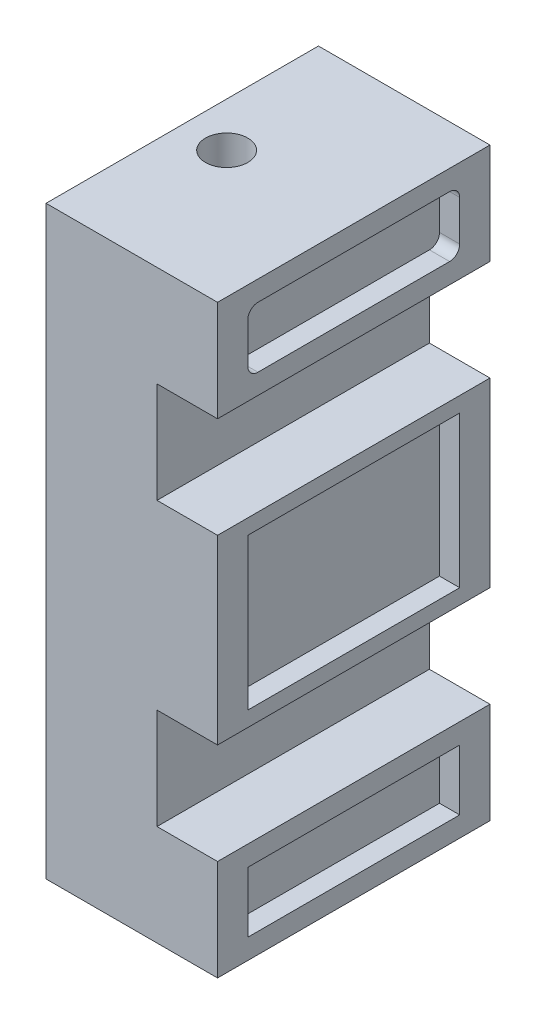
SolidWorks part; units mm, degrees
ref_plane "前视基准面" through (0, 0, 0) normal (0, 0, 1) x (1, 0, 0)
ref_plane "上视基准面" through (0, 0, 0) normal (0, 1, 0) x (1, 0, 0)
ref_plane "右视基准面" through (0, 0, 0) normal (1, 0, 0) x (0, 0, -1)
sketch "草图1" plane through (0, 0, 0) normal (0, 0, 1) x (1, 0, 0)
  line L0 (0, 0) -> (0, 29)
  line L1 (0, 29) -> (17, 29)
  line L2 (17, 29) -> (17, 19)
  line L3 (17, 19) -> (11, 19)
  line L4 (11, 19) -> (11, 9)
  line L5 (11, 9) -> (17, 9)
  line L6 (17, 9) -> (17, -9)
  line L7 (17, -9) -> (11, -9)
  line L8 (11, -9) -> (11, -19)
  line L9 (11, -19) -> (17, -19)
  line L10 (17, -19) -> (17, -29)
  line L11 (17, -29) -> (0, -29)
  line L12 (0, -29) -> (0, 0)
  dimension "D1" = 18
  dimension "D2" = 10
  dimension "D3" = 10
  dimension "D4" = 10
  dimension "D5" = 6
  dimension "D6" = 17
extrude "凸台-拉伸1" add sketch "草图1" along normal mid plane 27
sketch "草图2" plane through (17, 0, 0) normal (1, 0, 0) x (0, 0, -1)
  line L0 (-13.5, 29) -> (13.5, 29) construction
  line L1 (-10.5, 21) -> (10.5, 21)
  line L2 (-10.5, 21) -> (-10.5, 27)
  line L3 (-10.5, 27) -> (10.5, 27)
  line L4 (10.5, 21) -> (10.5, 27)
  line L5 (-10.5, 21) -> (10.5, 27) construction
  line L6 (-10.5, 27) -> (10.5, 21) construction
  line L7 (-13.5, 19) -> (13.5, 19) construction
  line L8 (13.5, 19) -> (13.5, 29) construction
  line L9 (-13.5, 19) -> (-13.5, 29) construction
  line L11 (-10.5, -7.5) -> (10.5, -7.5)
  line L12 (-10.5, -7.5) -> (-10.5, 7.5)
  line L13 (-10.5, 7.5) -> (10.5, 7.5)
  line L14 (10.5, -7.5) -> (10.5, 7.5)
  line L15 (-10.5, -7.5) -> (10.5, 7.5) construction
  line L16 (-10.5, 7.5) -> (10.5, -7.5) construction
  line L17 (-13.5, 9) -> (13.5, 9) construction
  line L18 (0, 0) -> (-13.5, 0) construction
  line L23 (-13.5, -9) -> (-13.5, 9) construction
  line L24 (-10.5, -27) -> (10.5, -21) construction
  line L25 (-10.5, -21) -> (10.5, -27) construction
  line L26 (10.5, -21) -> (10.5, -27)
  line L27 (-10.5, -27) -> (10.5, -27)
  line L28 (-10.5, -21) -> (-10.5, -27)
  line L29 (-10.5, -21) -> (10.5, -21)
  point P0 (0, 24)
  point P13 (0, 0)
  point P29 (0, -24)
  dimension "D1" = 2
  dimension "D2" = 2
  dimension "D3" = 3
  dimension "D4" = 3
  dimension "D5" = 1.5
extrude "切除-拉伸1" cut sketch "草图2" against normal blind 2
fillet "圆角1" radius 1 4 edges at (16, 27, 10.5) (16, 21, 10.5) (16, 21, -10.5) (16, 27, -10.5)
sketch "草图3" plane through (0, 29, 0) normal (0, 1, 0) x (1, 0, 0)
  line L0 (0, 0) -> (17, 0) construction
  line L1 (17, -13.5) -> (17, 13.5) construction
  line L2 (0, -13.5) -> (0, 13.5) construction
  circle A0 centre (4.4, 0) radius 2.1
  dimension "D1" = 4.2
  dimension "D2" = 4.4
extrude "切除-拉伸2" cut sketch "草图3" against normal up to surface (58 mm away) up to face at (8.5, -29, 0)
cosmetic thread "孔螺蚊线1" parameters "D1"=4, "D2"=5
sketch "草图5" plane through (0, 0, 0) normal (-1, 0, 0) x (0, 0, 1)
  circle A0 centre (0, 0) radius 2.1
  dimension "D1" = 4.2
extrude "切除-拉伸4" [suppressed] cut sketch "草图5" against normal up to next
hole_wizard "M5 螺纹孔1" positions "3D草图1" profile "草图6" tap size "M5" standard "GB"
sketch3d "3D草图1"
  circle A0 centre (4.4, 29, 0) radius 2.1 construction
  point P0 (4.4, 29, 0)
  point P5 (4.4, 31.1, 0)
sketch "草图6" plane through (4.4, 29, 0) normal (1, 0, 0) x (0, 0, 1)
  line L0 (0, 0) -> (0, 9.2618)
  line L1 (0, 9.2618) -> (2.1, 8)
  line L2 (2.1, 8) -> (2.1, 0)
  line L5 (2.1, 0) -> (0, 0)
  line L10 (0, 9.2618) -> (-2.1, 8) construction
  line L11 (0, -6.35) -> (0, 107.95) construction
  dimension "螺纹孔钻头直径" = 4.2
  dimension "螺纹孔钻头深度" = 8
  dimension "导头角度" = 118
